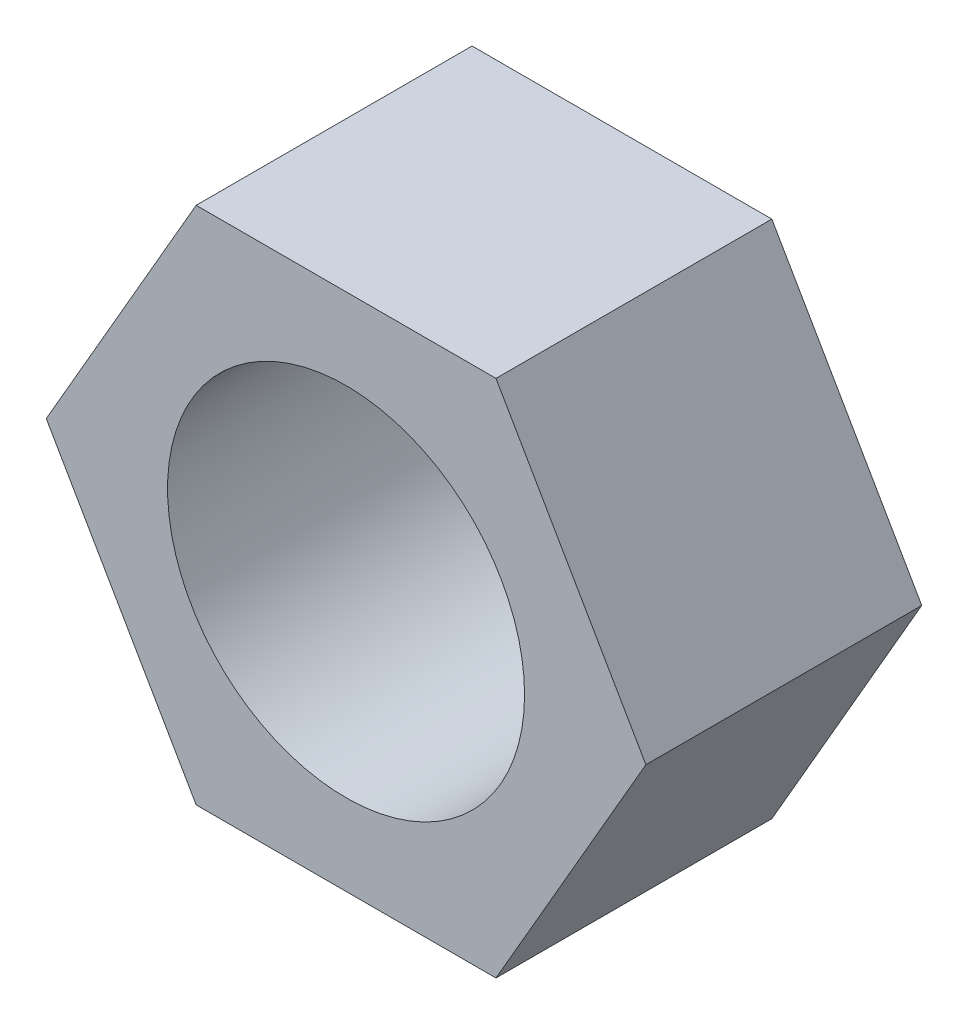
SolidWorks part; units mm, degrees
ref_plane "前视基准面" through (0, 0, 0) normal (0, 0, 1) x (1, 0, 0)
ref_plane "上视基准面" through (0, 0, 0) normal (0, 1, 0) x (1, 0, 0)
ref_plane "右视基准面" through (0, 0, 0) normal (1, 0, 0) x (0, 0, -1)
sketch "草图1" plane through (0, 0, 0) normal (0, 0, 1) x (1, 0, 0)
  line L1 (9.2376, 0) -> (4.6188, 8)
  line L2 (4.6188, 8) -> (-4.6188, 8)
  line L3 (-4.6188, 8) -> (-9.2376, 0)
  line L4 (-9.2376, 0) -> (-4.6188, -8)
  line L5 (-4.6188, -8) -> (4.6188, -8)
  line L6 (4.6188, -8) -> (9.2376, 0)
  circle A0 centre (0, 0) radius 8 construction
  dimension "D1" = 16
extrude "凸台-拉伸1" add sketch "草图1" along normal blind 8.5
sketch "草图2" plane through (0, 0, 8.5) normal (0, 0, 1) x (1, 0, 0)
  circle A0 centre (0, 0) radius 5.5
  dimension "D1" = 11
extrude "切除-拉伸1" cut sketch "草图2" against normal blind 8.5
